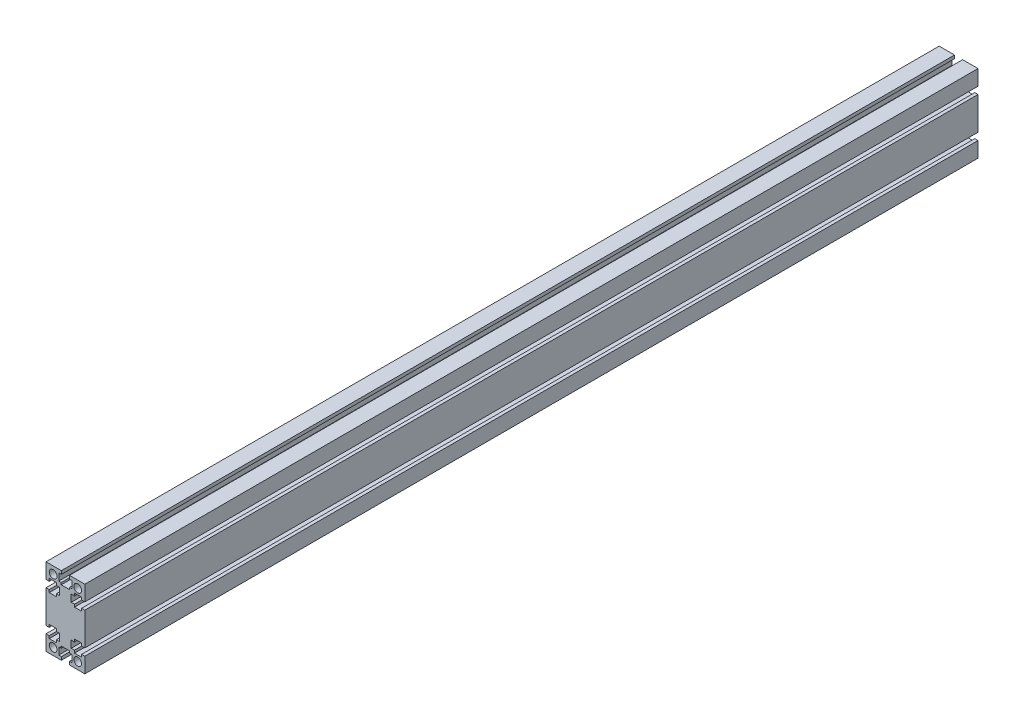
from build123d import *

# Parameters (mm, degrees)
SKETCH_1_R      = 3
EXTRUDE_1_DEPTH = 690


with BuildPart() as part:
    # 草图1 → 凸台-拉伸1 (new body)
    with BuildSketch(Plane.XY):
        Polygon((-27.495741056, 11.192504259), (-24.995741056, 11.192504259), (-24.995741056, 13.192504259), (-19.495741056, 13.192504259), (-19.495741056, 11.192504259), (-16.995741056, 11.192504259), (-16.995741056, 5.692504259), (-19.495741056, 5.692504259), (-19.495741056, 3.692504259), (-24.995741056, 3.692504259), (-24.995741056, 5.692504259), (-27.495741056, 5.692504259), (-27.495741056, -19.607495741), (-24.995741056, -19.607495741), (-24.995741056, -17.607495741), (-19.495741056, -17.607495741), (-19.495741056, -19.607495741), (-16.995741056, -19.607495741), (-16.995741056, -25.107495741), (-19.495741056, -25.107495741), (-19.495741056, -27.107495741), (-24.995741056, -27.107495741), (-24.995741056, -25.107495741), (-27.495741056, -25.107495741), (-27.495741056, -36.957495741), (-15.645741056, -36.957495741), (-15.645741056, -34.457495741), (-17.645741056, -34.457495741), (-17.645741056, -28.957495741), (-15.748076247, -28.957495741), (-15.748076247, -27.422563567), (-9.243405866, -27.422563567), (-9.243405866, -28.957495741), (-7.345741056, -28.957495741), (-7.345741056, -34.457495741), (-9.345741056, -34.457495741), (-9.345741056, -36.957495741), (2.504258944, -36.957495741), (2.504258944, -25.107495741), (0.004258944, -25.107495741), (0.004258944, -27.107495741), (-5.495741056, -27.107495741), (-5.495741056, -25.107495741), (-7.995741056, -25.107495741), (-7.995741056, -19.607495741), (-5.495741056, -19.607495741), (-5.495741056, -17.607495741), (0.004258944, -17.607495741), (0.004258944, -19.607495741), (2.504258944, -19.607495741), (2.504258944, 5.692504259), (0.004258944, 5.692504259), (0.004258944, 3.692504259), (-5.495741056, 3.692504259), (-5.495741056, 5.692504259), (-7.995741056, 5.692504259), (-7.995741056, 11.192504259), (-5.495741056, 11.192504259), (-5.495741056, 13.192504259), (0.004258944, 13.192504259), (0.004258944, 11.192504259), (2.504258944, 11.192504259), (2.504258944, 23.042504259), (-9.345741056, 23.042504259), (-9.345741056, 20.542504259), (-7.345741056, 20.542504259), (-7.345741056, 15.042504259), (-9.243405866, 15.042504259), (-9.243405866, 13.507572085), (-15.748076247, 13.507572085), (-15.748076247, 15.042504259), (-17.645741056, 15.042504259), (-17.645741056, 20.542504259), (-15.645741056, 20.542504259), (-15.645741056, 23.042504259), (-27.495741056, 23.042504259), align=None)
        with Locations((-21.995741056, 17.542504259)):
            Circle(SKETCH_1_R, mode=Mode.SUBTRACT)
        with Locations(Location((-2.995741056, 17.542504259, 0), (0, 0, 180))):
            Circle(SKETCH_1_R, mode=Mode.SUBTRACT)
        with Locations((-2.995741056, -31.457495741)):
            Circle(SKETCH_1_R, mode=Mode.SUBTRACT)
        with Locations(Location((-21.995741056, -31.457495741, 0), (0, 0, 180))):
            Circle(SKETCH_1_R, mode=Mode.SUBTRACT)
    extrude(amount=EXTRUDE_1_DEPTH)


solid = part.part
